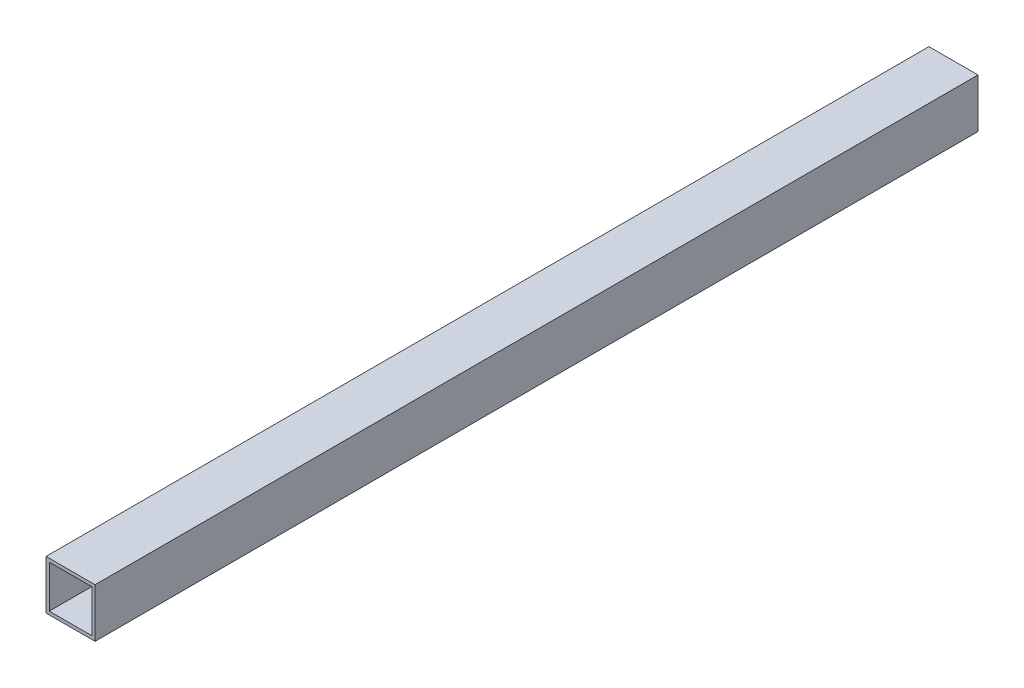
SolidWorks part; units mm, degrees
ref_plane "前视基准面" through (0, 0, 0) normal (0, 0, 1) x (1, 0, 0)
ref_plane "上视基准面" through (0, 0, 0) normal (0, 1, 0) x (1, 0, 0)
ref_plane "右视基准面" through (0, 0, 0) normal (1, 0, 0) x (0, 0, -1)
sketch "草图1" plane through (0, 0, 0) normal (0, 0, 1) x (1, 0, 0)
  line L0 (13, 13) -> (-13, 13)
  line L1 (15, -15) -> (-15, -15)
  line L2 (15, -15) -> (15, 15)
  line L3 (15, 15) -> (-15, 15)
  line L4 (-15, -15) -> (-15, 15)
  line L5 (15, -15) -> (-15, 15) construction
  line L6 (15, 15) -> (-15, -15) construction
  line L7 (-13, -13) -> (-13, 13)
  line L8 (13, -13) -> (-13, -13)
  line L9 (13, -13) -> (13, 13)
  point P0 (0, 0)
  dimension "D1" = 30
  dimension "D2" = 2
extrude "凸台-拉伸1" add sketch "草图1" along normal mid plane 540
sketch "草图2" plane through (0, 0, 270) normal (0, 0, 1) x (1, 0, 0)
  circle A0 centre (0, 0) radius 3.4
  point P12 (0, 0)
